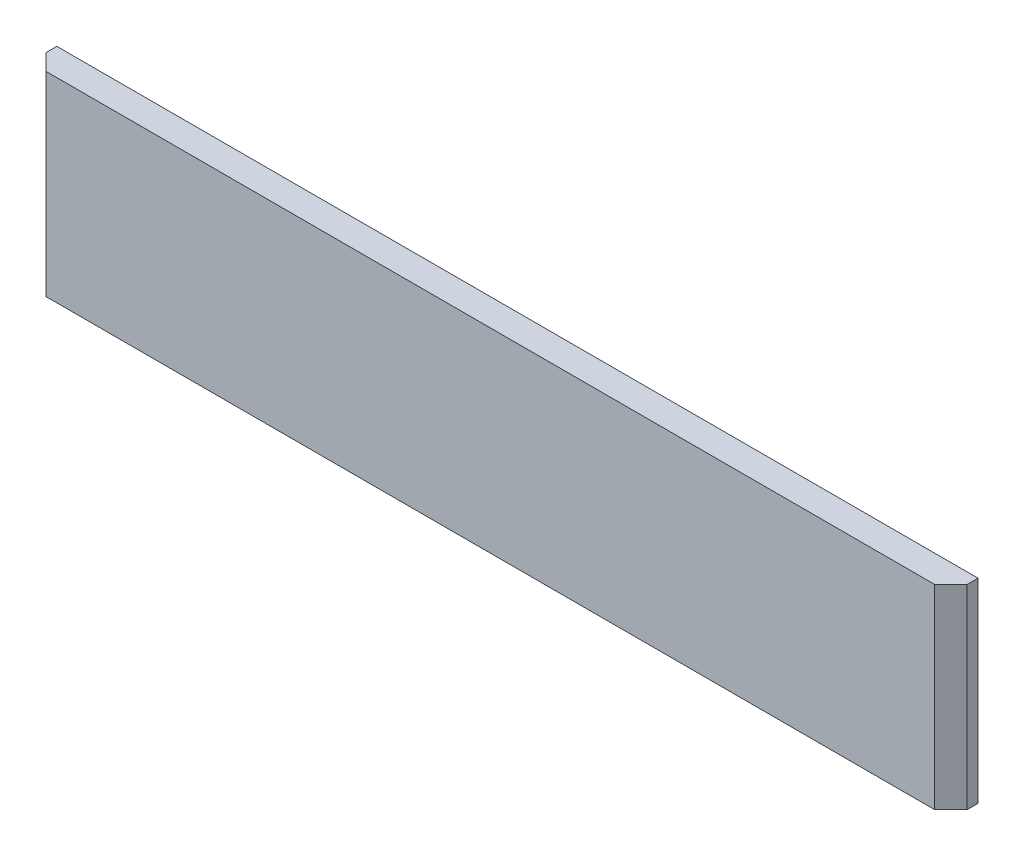
from build123d import *

# Parameters (mm, degrees)
SKETCH1_W           = 850
SKETCH1_H           = 180
BOSS_EXTRUDE1_DEPTH = 20
CHAMFER1_SIZE       = 15


with BuildPart() as part:
    # Sketch1 → Boss-Extrude1 (new, symmetric)
    with BuildSketch(Plane.XY):
        Rectangle(SKETCH1_W, SKETCH1_H)
    extrude(amount=BOSS_EXTRUDE1_DEPTH, both=True)

    # Chamfer1
    chamfer1_edges = [part.edges().sort_by_distance(p)[0] for p in [
        (425, 0, 20),
        (-425, 0, 20),
        (0, 90, -20),
        (425, 0, -20),
        (0, -90, -20),
        (-425, 0, -20),
    ]]
    chamfer(chamfer1_edges, length=CHAMFER1_SIZE)


solid = part.part
